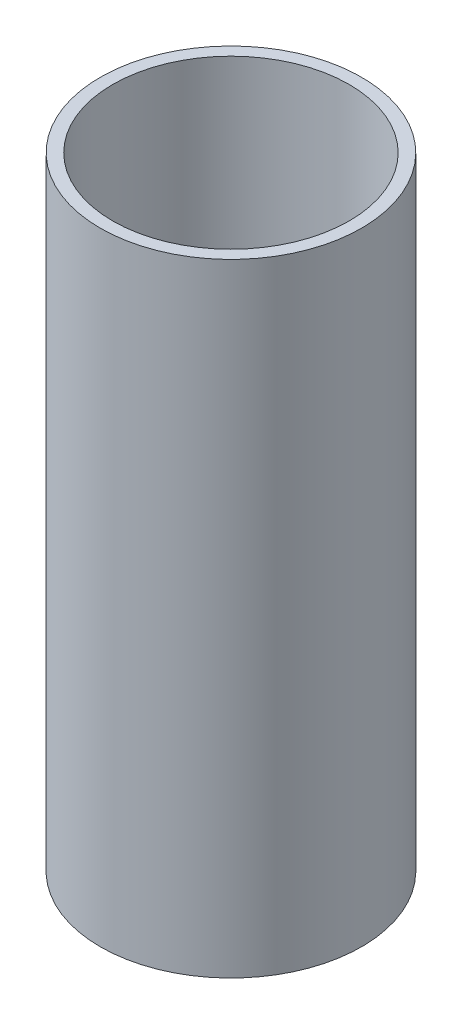
SolidWorks part; units mm, degrees
ref_plane "Front Plane" through (0, 0, 0) normal (0, 0, 1) x (1, 0, 0)
ref_plane "Top Plane" through (0, 0, 0) normal (0, 1, 0) x (1, 0, 0)
ref_plane "Right Plane" through (0, 0, 0) normal (1, 0, 0) x (0, 0, -1)
sketch "Sketch1" plane through (0, 0, 0) normal (0, 1, 0) x (1, 0, 0)
  circle A0 centre (0, 0) radius 10.5
  circle A1 centre (0, 0) radius 9.5
  dimension "D1" = 21
  dimension "D2" = 19
extrude "Boss-Extrude1" add sketch "Sketch1" along normal blind 50
